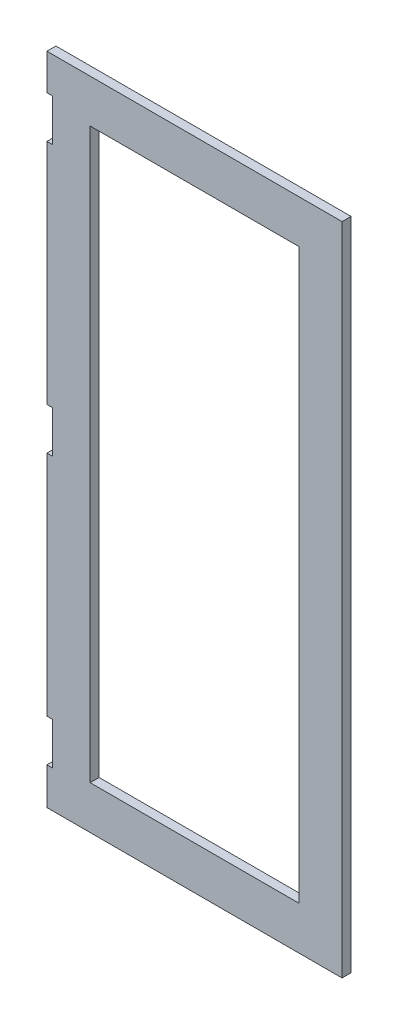
from build123d import *

# Parameters (mm, degrees)
SKETCH_1_W          = 820
SKETCH_1_H          = 1820
EXTRUDE_1_DEPTH     = 25
SKETCH_2_W          = 580
SKETCH_2_H          = 1580
CUT_EXTRUDE_1_DEPTH = 999.411237918
SKETCH_3_W          = 15
SKETCH_3_H          = 117
CUT_EXTRUDE_2_DEPTH = 999.411237918


with BuildPart() as part:
    # 草图1 → 凸台-拉伸1 (new body)
    with BuildSketch(Plane.XY):
        Rectangle(SKETCH_1_W, SKETCH_1_H)
    extrude(amount=EXTRUDE_1_DEPTH)

    # 草图2 → 切除-拉伸1 (cut, through all)
    with BuildSketch(Plane.XY.offset(25)):
        Rectangle(SKETCH_2_W, SKETCH_2_H)
    extrude(amount=-CUT_EXTRUDE_1_DEPTH, mode=Mode.SUBTRACT)

    # 草图3 → 切除-拉伸2 (cut, through all)
    with BuildSketch(Plane.XY.offset(25)):
        with Locations((-402.5, -748.5)):
            Rectangle(SKETCH_3_W, SKETCH_3_H)
        with Locations((-402.5, 1.5)):
            Rectangle(SKETCH_3_W, SKETCH_3_H)
        with Locations((-402.5, 751.5)):
            Rectangle(SKETCH_3_W, SKETCH_3_H)
    extrude(amount=-CUT_EXTRUDE_2_DEPTH, mode=Mode.SUBTRACT)


solid = part.part
